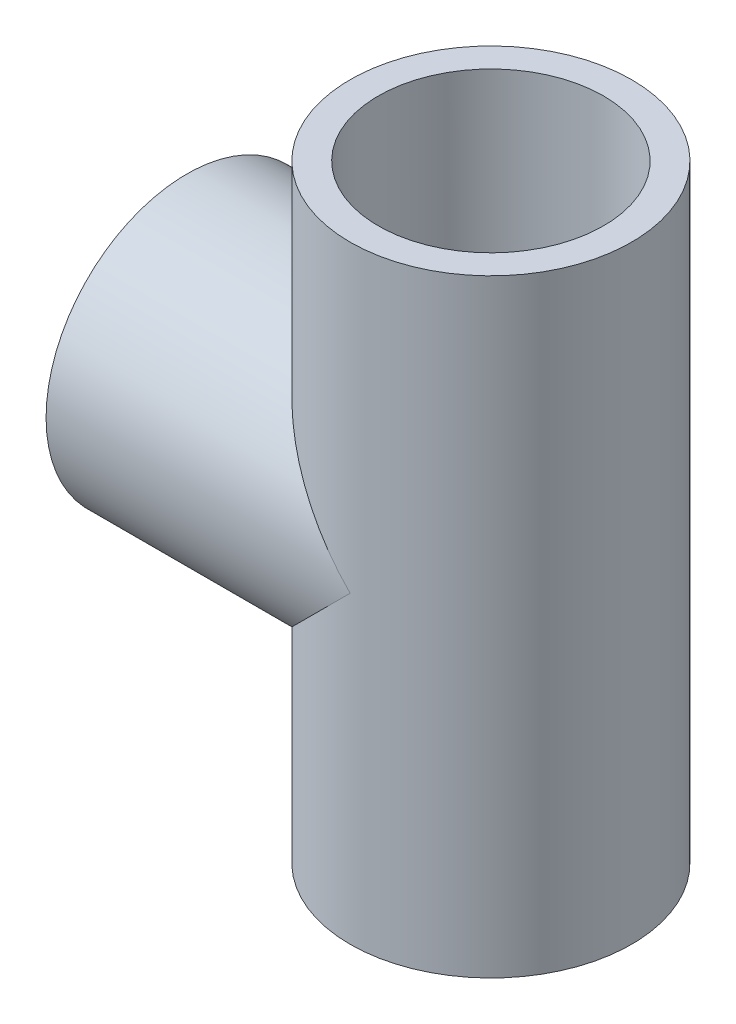
from build123d import *

# Parameters (mm, degrees)
SKETCH_1_W               = 2.5
SKETCH_1_H               = 27
PATTERN_CIRCULAR_1_COUNT = 3
PATTERN_CIRCULAR_1_ANGLE = 180
SKETCH_2_R               = 10
CUT_EXTRUDE_1_DEPTH      = 62.654278166
SKETCH_3_R               = 10
CUT_EXTRUDE_2_DEPTH      = 41.177730217


with BuildPart() as part:
    # 草图1 → 旋转1 (revolve)
    with BuildSketch(Plane.XY, mode=Mode.PRIVATE) as revolve_1_sk:
        with Locations((-11.25, 13.5)):
            Rectangle(SKETCH_1_W, SKETCH_1_H)
    revolve_1 = revolve(revolve_1_sk.sketch.rotate(Axis((0, 0, 0), (0, 1, 0)), 270), axis=Axis((0, 0, 0), (0, 1, 0)))

    # 阵列(圆周)1: 旋转1 ×3 about axis
    pattern_circular_1_axis = Axis((0, 0, 0), (0, 0, 1))
    for i in range(1, PATTERN_CIRCULAR_1_COUNT):
        add(revolve_1.rotate(pattern_circular_1_axis, i * PATTERN_CIRCULAR_1_ANGLE / (PATTERN_CIRCULAR_1_COUNT - 1)))

    # 草图2 → 切除-拉伸1 (cut, through all)
    with BuildSketch(Plane.XZ.offset(27)):
        with Locations(Location((0, 0, 0), (0, 0, 270))):
            Circle(SKETCH_2_R)
    extrude(amount=-CUT_EXTRUDE_1_DEPTH, mode=Mode.SUBTRACT)

    # 草图3 → 切除-拉伸2 (cut, through all)
    with BuildSketch(Plane(origin=(0, 0, 0), x_dir=(0, 0, -1), z_dir=(1, 0, 0))):
        Circle(SKETCH_3_R)
    extrude(amount=-CUT_EXTRUDE_2_DEPTH, mode=Mode.SUBTRACT)


solid = part.part
